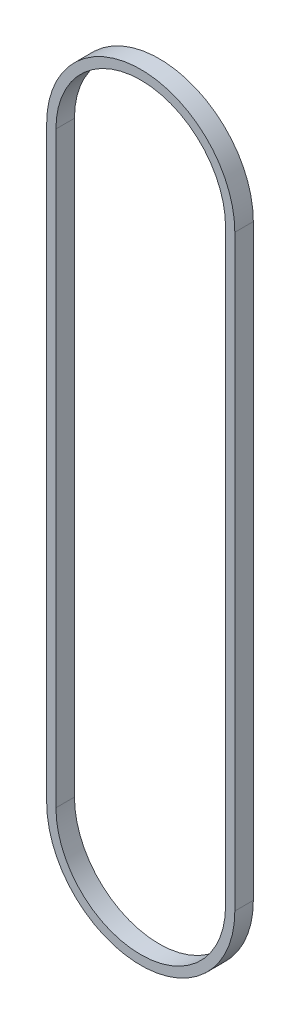
from build123d import *

# Parameters (mm, degrees)
EXTRUDE_1_DEPTH = 10


with BuildPart() as part:
    # 草图2 → 拉伸-薄壁1 (new, symmetric)
    with BuildSketch(Plane.XY):
        with BuildLine():
            Line((-101.625, -635), (-101.625, 0))
            ThreePointArc((-101.625, 0), (0, 101.625), (101.625, 0))
            Line((101.625, 0), (101.625, -635))
            ThreePointArc((101.625, -635), (0, -736.625), (-101.625, -635))
        make_face()
        with BuildLine():
            Line((-91.625, -635), (-91.625, 0))
            ThreePointArc((-91.625, 0), (0, 91.625), (91.625, 0))
            Line((91.625, 0), (91.625, -635))
            ThreePointArc((91.625, -635), (0, -726.625), (-91.625, -635))
        make_face(mode=Mode.SUBTRACT)
    extrude(amount=EXTRUDE_1_DEPTH, both=True)


solid = part.part
